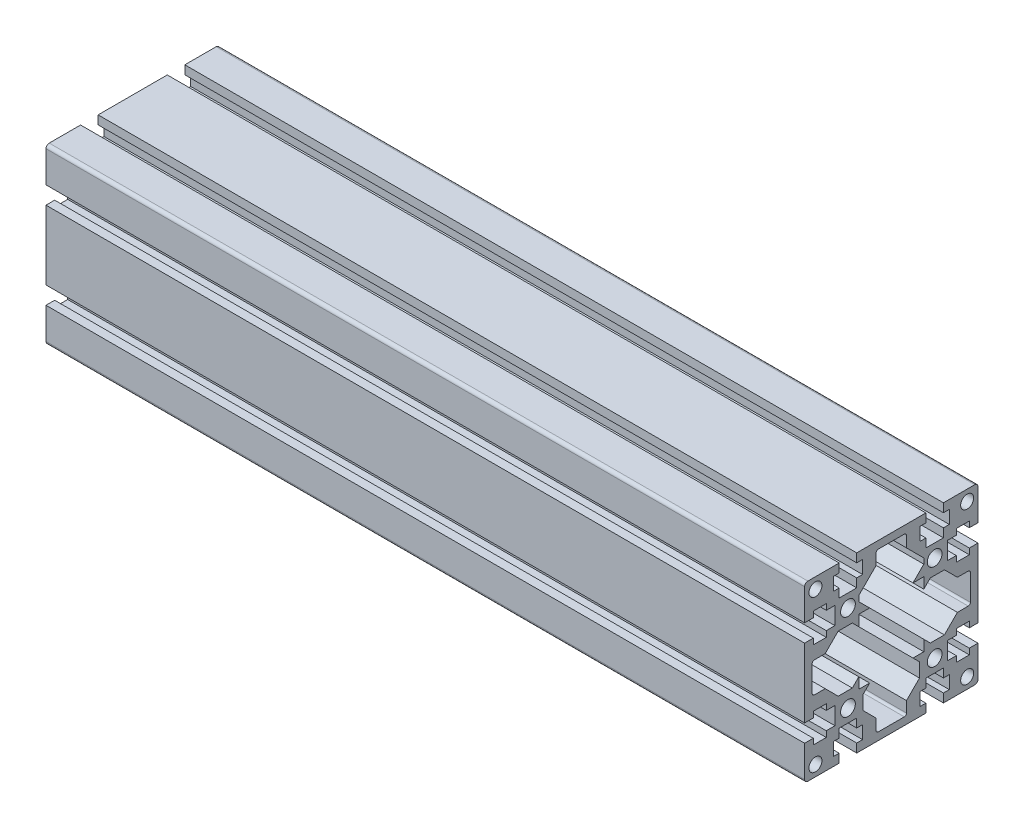
from build123d import *

# Parameters (mm, degrees)
SKETCH1_R                                 = 3.4
SKETCH1_R_2                               = 3
ALUMINIUM_PROFILE_80_X_80G_X_R1_5_1_DEPTH = 350
SKETCH10_R                                = 3
CUT_EXTRUDE1_DEPTH                        = 355.541958025


with BuildPart() as part:
    # Sketch1 → Aluminium profile 80 X 80G X R1.5(1) (new body)
    with BuildSketch(Plane.YZ.offset(-530.344827586)):
        with BuildLine():
            Line((-24.05, 40), (-24.05, 36))
            Line((-24.05, 36), (-26.75, 36))
            Line((-26.75, 36), (-26.75, 30))
            Line((-26.75, 30), (-24.05, 30))
            Line((-24.05, 30), (-24.05, 26))
            Line((-24.05, 26), (-15.95, 26))
            Line((-15.95, 26), (-15.95, 30))
            Line((-15.95, 30), (-13.25, 30))
            Line((-13.25, 30), (-13.25, 36))
            Line((-13.25, 36), (-15.95, 36))
            Line((-15.95, 36), (-15.95, 40))
            Line((-15.95, 40), (15.95, 40))
            Line((15.95, 40), (15.95, 36))
            Line((15.95, 36), (13.25, 36))
            Line((13.25, 36), (13.25, 30))
            Line((13.25, 30), (15.95, 30))
            Line((15.95, 30), (15.95, 26))
            Line((15.95, 26), (24.05, 26))
            Line((24.05, 26), (24.05, 30))
            Line((24.05, 30), (26.75, 30))
            Line((26.75, 30), (26.75, 36))
            Line((26.75, 36), (24.05, 36))
            Line((24.05, 36), (24.05, 40))
            Line((24.05, 40), (38.5, 40))
            ThreePointArc((38.5, 40), (39.560660172, 39.560660172), (40, 38.5))
            Line((40, 38.5), (40, 24.05))
            Line((40, 24.05), (36, 24.05))
            Line((36, 24.05), (36, 26.75))
            Line((36, 26.75), (30, 26.75))
            Line((30, 26.75), (30, 24.05))
            Line((30, 24.05), (26, 24.05))
            Line((26, 24.05), (26, 15.95))
            Line((26, 15.95), (30, 15.95))
            Line((30, 15.95), (30, 13.25))
            Line((30, 13.25), (36, 13.25))
            Line((36, 13.25), (36, 15.95))
            Line((36, 15.95), (40, 15.95))
            Line((40, 15.95), (40, -15.95))
            Line((40, -15.95), (36, -15.95))
            Line((36, -15.95), (36, -13.25))
            Line((36, -13.25), (30, -13.25))
            Line((30, -13.25), (30, -15.95))
            Line((30, -15.95), (26, -15.95))
            Line((26, -15.95), (26, -24.05))
            Line((26, -24.05), (30, -24.05))
            Line((30, -24.05), (30, -26.75))
            Line((30, -26.75), (36, -26.75))
            Line((36, -26.75), (36, -24.05))
            Line((36, -24.05), (40, -24.05))
            Line((40, -24.05), (40, -38.5))
            ThreePointArc((40, -38.5), (39.560660172, -39.560660172), (38.5, -40))
            Line((38.5, -40), (24.05, -40))
            Line((24.05, -40), (24.05, -36))
            Line((24.05, -36), (26.75, -36))
            Line((26.75, -36), (26.75, -30))
            Line((26.75, -30), (24.05, -30))
            Line((24.05, -30), (24.05, -26))
            Line((24.05, -26), (15.95, -26))
            Line((15.95, -26), (15.95, -30))
            Line((15.95, -30), (13.25, -30))
            Line((13.25, -30), (13.25, -36))
            Line((13.25, -36), (15.95, -36))
            Line((15.95, -36), (15.95, -40))
            Line((15.95, -40), (-15.95, -40))
            Line((-15.95, -40), (-15.95, -36))
            Line((-15.95, -36), (-13.25, -36))
            Line((-13.25, -36), (-13.25, -30))
            Line((-13.25, -30), (-15.95, -30))
            Line((-15.95, -30), (-15.95, -26))
            Line((-15.95, -26), (-24.05, -26))
            Line((-24.05, -26), (-24.05, -30))
            Line((-24.05, -30), (-26.75, -30))
            Line((-26.75, -30), (-26.75, -36))
            Line((-26.75, -36), (-24.05, -36))
            Line((-24.05, -36), (-24.05, -40))
            Line((-24.05, -40), (-38.5, -40))
            ThreePointArc((-38.5, -40), (-39.560660172, -39.560660172), (-40, -38.5))
            Line((-40, -38.5), (-40, -24.05))
            Line((-40, -24.05), (-36, -24.05))
            Line((-36, -24.05), (-36, -26.75))
            Line((-36, -26.75), (-30, -26.75))
            Line((-30, -26.75), (-30, -24.05))
            Line((-30, -24.05), (-26, -24.05))
            Line((-26, -24.05), (-26, -15.95))
            Line((-26, -15.95), (-30, -15.95))
            Line((-30, -15.95), (-30, -13.25))
            Line((-30, -13.25), (-36, -13.25))
            Line((-36, -13.25), (-36, -15.95))
            Line((-36, -15.95), (-40, -15.95))
            Line((-40, -15.95), (-40, 15.95))
            Line((-40, 15.95), (-36, 15.95))
            Line((-36, 15.95), (-36, 13.25))
            Line((-36, 13.25), (-30, 13.25))
            Line((-30, 13.25), (-30, 15.95))
            Line((-30, 15.95), (-26, 15.95))
            Line((-26, 15.95), (-26, 24.05))
            Line((-26, 24.05), (-30, 24.05))
            Line((-30, 24.05), (-30, 26.75))
            Line((-30, 26.75), (-36, 26.75))
            Line((-36, 26.75), (-36, 24.05))
            Line((-36, 24.05), (-40, 24.05))
            Line((-40, 24.05), (-40, 38.5))
            ThreePointArc((-40, 38.5), (-39.560660172, 39.560660172), (-38.5, 40))
            Line((-38.5, 40), (-24.05, 40))
        make_face()
        with Locations((-20, 20)):
            Circle(SKETCH1_R, mode=Mode.SUBTRACT)
        with Locations((20, 20)):
            Circle(SKETCH1_R, mode=Mode.SUBTRACT)
        with Locations((20, -20)):
            Circle(SKETCH1_R, mode=Mode.SUBTRACT)
        with Locations((-20, -20)):
            Circle(SKETCH1_R, mode=Mode.SUBTRACT)
        with Locations((-35, 35)):
            Circle(SKETCH1_R_2, mode=Mode.SUBTRACT)
        with Locations((35, 35)):
            Circle(SKETCH1_R_2, mode=Mode.SUBTRACT)
        with Locations((35, -35)):
            Circle(SKETCH1_R_2, mode=Mode.SUBTRACT)
        with BuildLine():
            Line((-13, 18), (-10, 15))
            Line((-10, 15), (-15, 15))
            Line((-15, 15), (-15, 10))
            Line((-15, 10), (-18, 13))
            Line((-18, 13), (-24.5, 13))
            Line((-24.5, 13), (-30.5, 7))
            Line((-30.5, 7), (-35.5, 7))
            ThreePointArc((-35.5, 7), (-36.207106781, 6.707106781), (-36.5, 6))
            Line((-36.5, 6), (-36.5, -6))
            ThreePointArc((-36.5, -6), (-36.207106781, -6.707106781), (-35.5, -7))
            Line((-35.5, -7), (-30.5, -7))
            Line((-30.5, -7), (-24.5, -13))
            Line((-24.5, -13), (-18, -13))
            Line((-18, -13), (-15, -10))
            Line((-15, -10), (-15, -15))
            Line((-15, -15), (-10, -15))
            Line((-10, -15), (-13, -18))
            Line((-13, -18), (-13, -24.5))
            Line((-13, -24.5), (-7, -30.5))
            Line((-7, -30.5), (-7, -35.5))
            ThreePointArc((-7, -35.5), (-6.707106781, -36.207106781), (-6, -36.5))
            Line((-6, -36.5), (6, -36.5))
            ThreePointArc((6, -36.5), (6.707106781, -36.207106781), (7, -35.5))
            Line((7, -35.5), (7, -30.5))
            Line((7, -30.5), (13, -24.5))
            Line((13, -24.5), (13, -18))
            Line((13, -18), (10, -15))
            Line((10, -15), (15, -15))
            Line((15, -15), (15, -10))
            Line((15, -10), (20, -15))
            Line((20, -15), (22.5, -15))
            Line((22.5, -15), (30.5, -7))
            Line((30.5, -7), (35.5, -7))
            ThreePointArc((35.5, -7), (36.207106781, -6.707106781), (36.5, -6))
            Line((36.5, -6), (36.5, 6))
            ThreePointArc((36.5, 6), (36.207106781, 6.707106781), (35.5, 7))
            Line((35.5, 7), (30.5, 7))
            Line((30.5, 7), (22.5, 15))
            Line((22.5, 15), (20, 15))
            Line((20, 15), (15, 10))
            Line((15, 10), (15, 15))
            Line((15, 15), (10, 15))
            Line((10, 15), (13, 18))
            Line((13, 18), (13, 24.5))
            Line((13, 24.5), (7, 30.5))
            Line((7, 30.5), (7, 35.5))
            ThreePointArc((7, 35.5), (6.707106781, 36.207106781), (6, 36.5))
            Line((6, 36.5), (-6, 36.5))
            ThreePointArc((-6, 36.5), (-6.707106781, 36.207106781), (-7, 35.5))
            Line((-7, 35.5), (-7, 30.5))
            Line((-7, 30.5), (-13, 24.5))
            Line((-13, 24.5), (-13, 18))
        make_face(mode=Mode.SUBTRACT)
    extrude(amount=ALUMINIUM_PROFILE_80_X_80G_X_R1_5_1_DEPTH)

    # Sketch10 → Cut-Extrude1 (cut, through all)
    with BuildSketch(Plane(origin=(-180.344827586, 0, 0), x_dir=(0, 0, -1), z_dir=(1, 0, 0))):
        with Locations((35, -35)):
            Circle(SKETCH10_R)
    extrude(amount=-CUT_EXTRUDE1_DEPTH, mode=Mode.SUBTRACT)


solid = part.part
